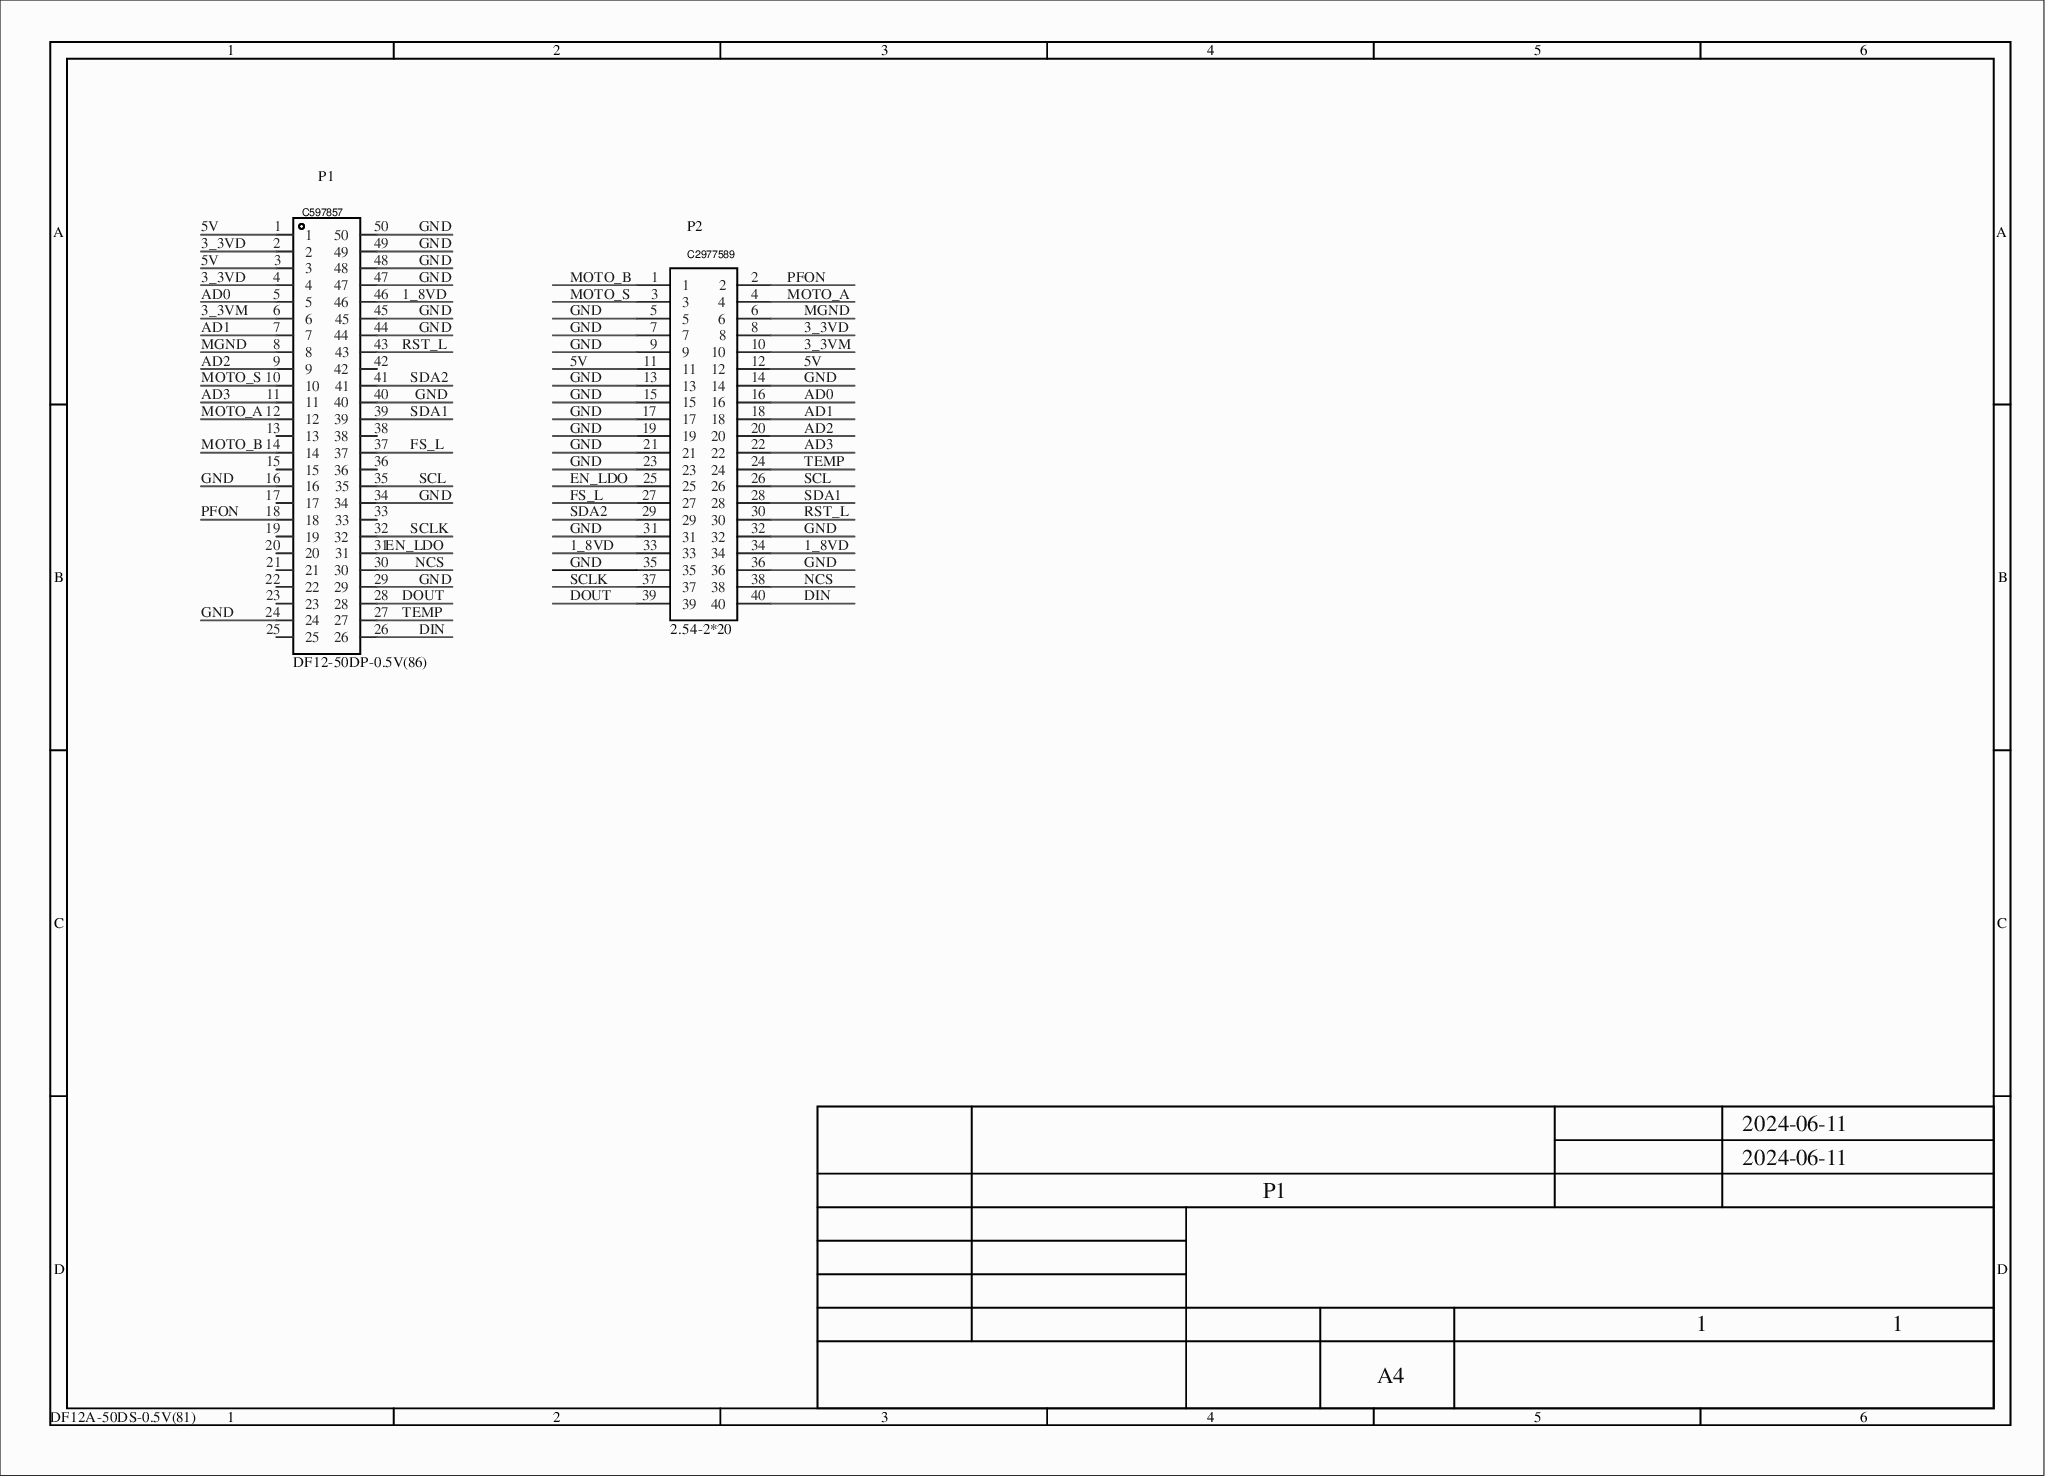
[diagram p0: MISC89329-2.schdoc]
# Altium project MISC89329-8.PrjPCB
1 sheet, 2 parts. Net scope: global (net labels, ports and power ports of the same name join across sheets).
Board file: MISC89329.PcbDoc

## Sheet MISC89329-2.schdoc
size 309 x 223 mm; Version: V1.0; @Project Name: MISC89329; @Page Count: 1; @Update Date: 2024-06-11; @Create Date: 2024-06-11; @Schematic Name: MISC89329; @Page No: 1

### Parts
P1  Name: DF12-50DP-0.5V(86)  Supplier Part: C597857  [CONN-SMD_DF12A-3.0-50DS-0.5]  (hidden comment: DF12A-50DS-0.5V(81))
P2  Supplier Part: C2977589  [HDR-TH_40P-P2.54-V-F-R2-C20-S2.54]  (hidden comment: 2.54-2*20)

### Nets
1_8VD: P1.46 P2.33 P2.34
3_3VD: P1.2 P1.4 P2.8
3_3VM: P1.6 P2.10
5V: P1.1 P1.3 P2.11 P2.12
AD0: P1.5 P2.16
AD1: P1.7 P2.18
AD2: P1.9 P2.20
AD3: P1.11 P2.22
DIN: P1.26 P2.40
DOUT: P1.28 P2.39
EN_LDO: P1.31 P2.25
FS_L: P1.37 P2.27
GND: P1.16 P1.24 P1.29 P1.34 P1.40 P1.44 P1.45 P1.47 P1.48 P1.49 P1.50 P2.5 P2.7 P2.9 P2.13 P2.14 P2.15 P2.17 P2.19 P2.21 P2.23 P2.31 P2.32 P2.35 P2.36
MGND: P1.8 P2.6
MOTO_A: P1.12 P2.4
MOTO_B: P1.14 P2.1
MOTO_S: P1.10 P2.3
NCS: P1.30 P2.38
PFON: P1.18 P2.2
RST_L: P1.43 P2.30
SCL: P1.35 P2.26
SCLK: P1.32 P2.37
SDA1: P1.39 P2.28
SDA2: P1.41 P2.29
TEMP: P1.27 P2.24

Not connected (* = marked no-connect by the designer): P1 13 15 17 19 20 21 22 23 25 33 36 38 42

### Notes on the sheet
- 1
- 2
- 3
- 4
- 5
- 6
- A
- B
- C
- 2024-06-11
- P1
- D
- A4

### Library data of the parts
P1 = DF12A-50DS-0.5V(81): Add into BOM: yes; Pitch: 0.5mm; Current Rating (Max): 300mA; Symbol: DF12A-50DS-0.5V(81); Device: DF12A-50DS-0.5V(81); Manufacturer Part: DF12A-50DS-0.5V(81); Supplier Footprint: SMD,P=0.5mm; Datasheet: https://example.com/upload/public/pdf/source/20200611/C597843_9BBDCF5791D5AB21AB74AD82BADE88A8.pdf; Supplier: LCSC; Convert to PCB: yes; Number of Pins: 50P; Number of Rows: 2
P2 = 2.54-2*20: Add into BOM: yes; Holes Structure: 2x20P; Pitch: 2.54mm; Number of Holes: 40P; Current Rating (Max): 2.5A; Name: 2.54-2*20; Symbol: 2.54-2*20; Device: 2.54-2*20; Manufacturer Part: 2.54-2*20; Datasheet: https://example.com/upload/public/pdf/source/20220328/834E302BE3C038BBC5C70F5E02589B1E.pdf; Supplier: LCSC; Convert to PCB: yes; Row Spacing: 2.54mm; Voltage Rating (Max): -; Insulation Height: 8.5mm